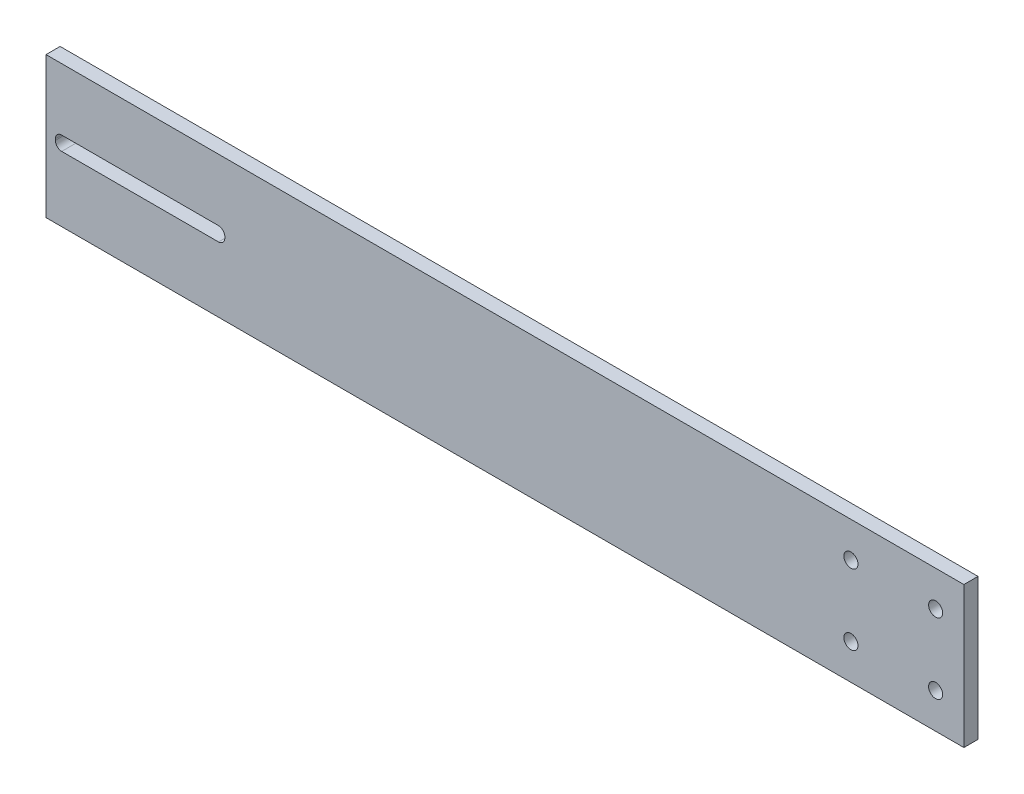
SolidWorks part; units mm, degrees
material "PVC Rigid"
ref_plane "Front Plane" through (0, 0, 0) normal (0, 0, 1) x (1, 0, 0)
ref_plane "Top Plane" through (0, 0, 0) normal (0, 1, 0) x (1, 0, 0)
ref_plane "Right Plane" through (0, 0, 0) normal (1, 0, 0) x (0, 0, -1)
sketch "Sketch1" plane through (0, 0, 0) normal (0, 0, 1) x (1, 0, 0)
  line L1 (325, -50) -> (-325, -50)
  line L2 (325, -50) -> (325, 50)
  line L3 (325, 50) -> (-325, 50)
  line L4 (-325, -50) -> (-325, 50)
  line L5 (325, -50) -> (-325, 50) construction
  line L6 (325, 50) -> (-325, -50) construction
  point P0 (0, 0)
  dimension "D1" = 650
  dimension "D2" = 100
extrude "Boss-Extrude1" add sketch "Sketch1" along normal blind 10
sketch "Sketch2" plane through (0, 0, 10) normal (0, 0, 1) x (1, 0, 0)
  line L0 (342.8565, 0) -> (125.906, 0) construction
  line L1 (335.6409, 25) -> (151.8823, 25) construction
  line L2 (354.8826, -25) -> (151.8823, -25) construction
  line L3 (325, -50) -> (325, 50) construction
  circle A0 centre (305, 25) radius 5
  circle A1 centre (245, 25) radius 5
  circle A2 centre (245, -25) radius 5
  circle A3 centre (305, -25) radius 5
  dimension "D3" = 10
  dimension "D4" = 10
  dimension "D5" = 10
  dimension "D6" = 10
  dimension "D1" = 25
  dimension "D2" = 25
  dimension "D7" = 20
  dimension "D8" = 20
  dimension "D9" = 60
  dimension "D10" = 60
extrude "Cut-Extrude2" cut sketch "Sketch2" against normal blind 10
sketch "Sketch3" plane through (0, 0, 10) normal (0, 0, 1) x (1, 0, 0)
  line L1 (-313.885, -3.8143) -> (-202.885, -3.8143)
  line L2 (-318.385, 0.6857) -> (-318.385, 1.6857)
  line L3 (-313.885, 6.1857) -> (-202.885, 6.1857)
  line L4 (-198.385, 0.6857) -> (-198.385, 1.6857)
  line L5 (-318.385, -3.8143) -> (-198.385, 6.1857) construction
  line L6 (-318.385, 6.1857) -> (-198.385, -3.8143) construction
  arc A0 (-202.885, -3.8143) -> (-198.385, 0.6857) centre (-202.885, 0.6857) ccw
  arc A1 (-202.885, 6.1857) -> (-198.385, 1.6857) centre (-202.885, 1.6857) cw
  arc A2 (-313.885, -3.8143) -> (-318.385, 0.6857) centre (-313.885, 0.6857) cw
  arc A3 (-318.385, 1.6857) -> (-313.885, 6.1857) centre (-313.885, 1.6857) cw
  point P0 (-258.385, 1.1857)
  dimension "D3" = 4.5
  dimension "D1" = 120
  dimension "D2" = 10
extrude "Cut-Extrude3" cut sketch "Sketch3" against normal blind 10
